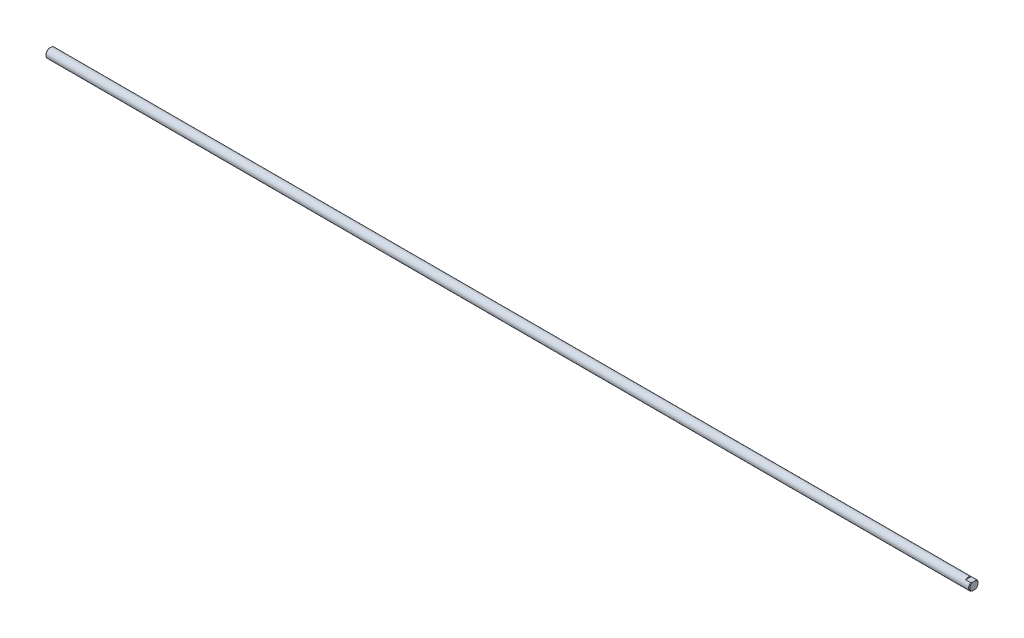
from build123d import *

# Parameters (mm, degrees)
SKETCH1_R               = 7.5
BOSS_EXTRUDE1_DEPTH     = 1480
CHAMFER1_SIZE           = 1
CUT_EXTRUDE1_DEPTH      = 1481.038006269
CUT_EXTRUDE1_DEPTH_BACK = 1481.038006269
SKETCH8_W               = 43.567276196
SKETCH8_H               = 1.89956865


with BuildPart() as part:
    # Sketch1 → Boss-Extrude1 (new body)
    with BuildSketch(Plane(origin=(0, 0, 0), x_dir=(0, 0, -1), z_dir=(1, 0, 0))):
        Circle(SKETCH1_R)
    extrude(amount=BOSS_EXTRUDE1_DEPTH)

    # Chamfer1
    chamfer1_edges = [part.edges().sort_by_distance(p)[0] for p in [
        (0, 0, 7.5),
        (1480, 0, 7.5),
    ]]
    chamfer(chamfer1_edges, length=CHAMFER1_SIZE)

    # Sketch8 → Cut-Extrude1 (cut, two sides: drawn at the far end of the back side and taken through both)
    with BuildSketch(Plane.XY.offset(-CUT_EXTRUDE1_DEPTH_BACK)):
        with Locations((1492.783638098, 6.949784325)):
            Rectangle(SKETCH8_W, SKETCH8_H)
        with Locations((1492.783638098, -6.949784325)):
            Rectangle(SKETCH8_W, SKETCH8_H)
    extrude(amount=CUT_EXTRUDE1_DEPTH + CUT_EXTRUDE1_DEPTH_BACK, mode=Mode.SUBTRACT)


solid = part.part
